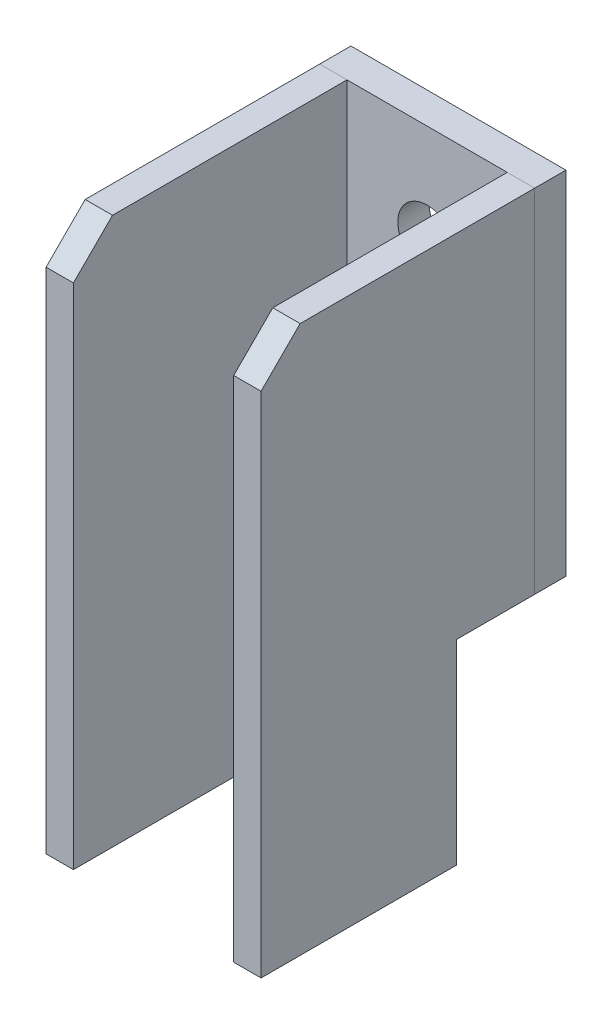
from build123d import *

# Parameters (mm, degrees)
SKETCH_1_W          = 110
SKETCH_1_H          = 100
EXTRUDE_1_DEPTH     = 16
EXTRUDE_2_DEPTH     = 14
CHAMFER_1_SIZE      = 20
SKETCH_3_R          = 15
CUT_EXTRUDE_1_DEPTH = 16
SKETCH_4_W          = 110
SKETCH_4_H          = 16
EXTRUDE_3_DEPTH     = 80


with BuildPart() as part:
    # 草图1 → 凸台-拉伸1 (new body)
    with BuildSketch(Plane.XY):
        Rectangle(SKETCH_1_W, SKETCH_1_H)
    extrude(amount=EXTRUDE_1_DEPTH)

    # 草图3 → 切除-拉伸1 (cut)
    with BuildSketch(Plane(origin=(0, 0, 0), x_dir=(-1, 0, 0), z_dir=(0, 0, -1))):
        Circle(SKETCH_3_R)
    extrude(amount=-CUT_EXTRUDE_1_DEPTH, mode=Mode.SUBTRACT)

    # 草图4 → 凸台-拉伸3 (add)
    with BuildSketch(Plane.XZ.offset(50)):
        with Locations((0, 8)):
            Rectangle(SKETCH_4_W, SKETCH_4_H)
    extrude(amount=EXTRUDE_3_DEPTH)


with BuildPart() as body_2:
    # 草图2 → 凸台-拉伸2 (new body)
    with BuildSketch(Plane.ZY.offset(55)):
        Polygon((16, 50), (16, -130), (56, -130), (56, -230), (156, -230), (156, 50), align=None)
    extrude(amount=-EXTRUDE_2_DEPTH)

    # 倒角1
    chamfer_1_edges = [body_2.edges().sort_by_distance(p)[0] for p in [
        (-48, 50, 156),
    ]]
    chamfer(chamfer_1_edges, length=CHAMFER_1_SIZE)


with BuildPart() as body_3:
    # 镜向1: mirrored copy
    add(body_2.part.mirror(Plane(origin=(0, 0, 0), x_dir=(0, 0, 1), z_dir=(1, 0, 0))))


solid = Compound([part.part, body_2.part, body_3.part])
